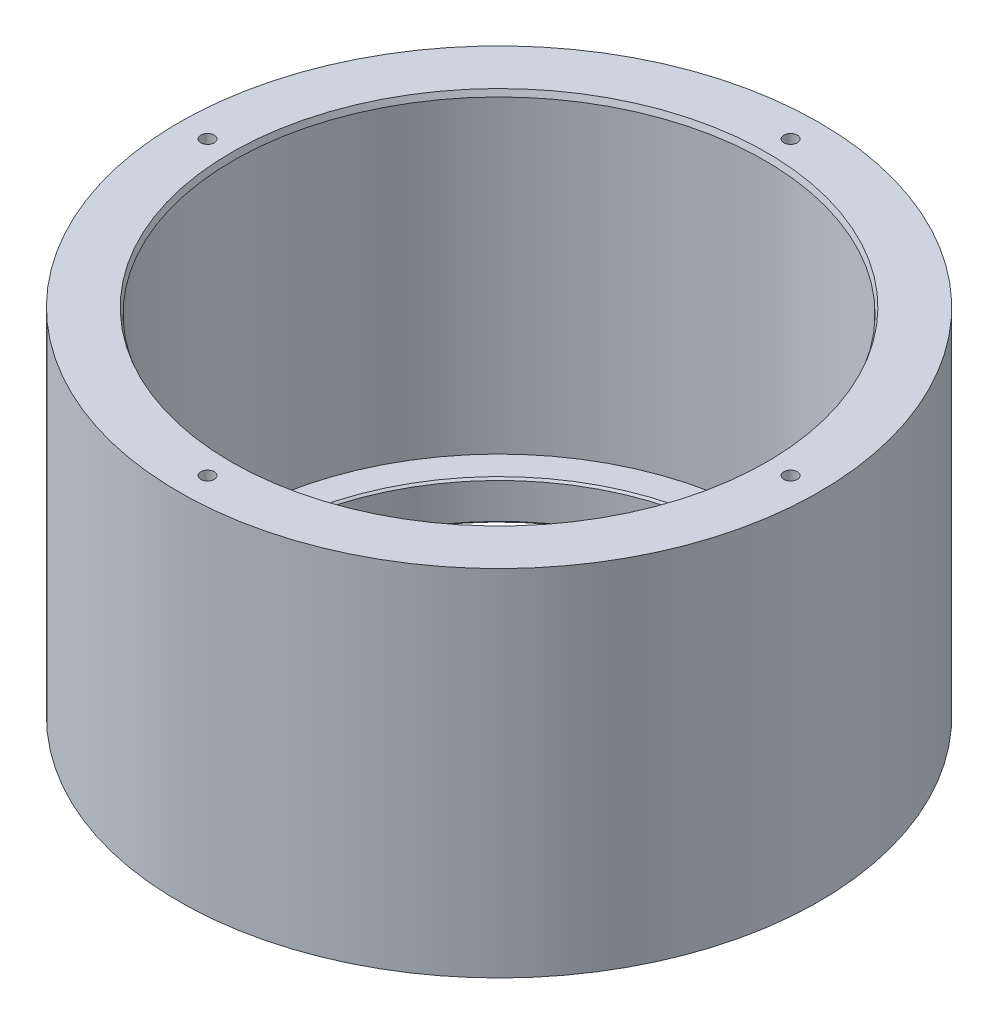
from build123d import *

# Parameters (mm, degrees)
SKETCH1_R             = 162.5
SKETCH1_R_2           = 120
BOSS_EXTRUDE1_DEPTH   = 180
SKETCH2_R             = 135
CUT_EXTRUDE1_DEPTH    = 160
CHAMFER1_SIZE         = 1
CHAMFER1_SIZE2        = 3
CHAMFER2_SIZE         = 1
M8_TAPPED_HOLE1_D     = 6.8
M8_TAPPED_HOLE1_DEPTH = 26
M8_TAPPED_HOLE1_TIP   = 2.042926105


with BuildPart() as part:
    # Sketch1 → Boss-Extrude1 (new body)
    with BuildSketch(Plane(origin=(0, 0, 0), x_dir=(1, 0, 0), z_dir=(0, 1, 0))):
        with Locations(Location((0, 0, 0), (0, 0, 90))):
            Circle(SKETCH1_R)
        with Locations(Location((0, 0, 0), (0, 0, 90))):
            Circle(SKETCH1_R_2, mode=Mode.SUBTRACT)
    extrude(amount=BOSS_EXTRUDE1_DEPTH)

    # Sketch2 → Cut-Extrude1 (cut)
    with BuildSketch(Plane(origin=(0, 180, 0), x_dir=(1, 0, 0), z_dir=(0, 1, 0))):
        with Locations(Location((0, 0, 0), (0, 0, 270))):
            Circle(SKETCH2_R)
    extrude(amount=-CUT_EXTRUDE1_DEPTH, mode=Mode.SUBTRACT)

    # Chamfer1
    chamfer1_edges = [part.edges().sort_by_distance(p)[0] for p in [
        (0, 180, -135),
    ]]
    chamfer1_side = [part.faces().sort_by_distance(p)[0] for p in [
        (0, 180, 157.903805922),
    ]]
    chamfer(chamfer1_edges, length=CHAMFER1_SIZE, length2=CHAMFER1_SIZE2, reference=chamfer1_side[0])

    # Chamfer2
    chamfer2_edges = [part.edges().sort_by_distance(p)[0] for p in [
        (0, 20, 120),
        (0, 0, 120),
    ]]
    chamfer(chamfer2_edges, length=CHAMFER2_SIZE)

    # M8 Tapped Hole1
    with Locations(Plane(origin=(0, 180, 0), x_dir=(1, 0, 0), z_dir=(0, 1, 0))):
        with Locations((148, 0), (0, -148), (-148, 0), (0, 148)):
            Hole(M8_TAPPED_HOLE1_D / 2, depth=M8_TAPPED_HOLE1_DEPTH)
            with Locations((0, 0, -(M8_TAPPED_HOLE1_DEPTH + M8_TAPPED_HOLE1_TIP / 2))):  # 118° drill point
                Cone(0, M8_TAPPED_HOLE1_D / 2, M8_TAPPED_HOLE1_TIP, mode=Mode.SUBTRACT)


solid = part.part
